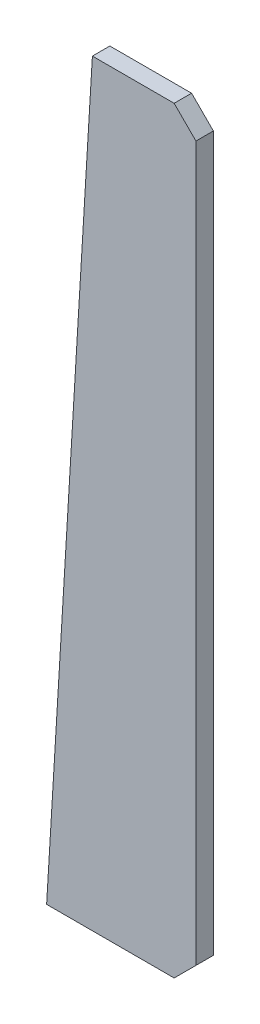
from build123d import *

# Parameters (mm, degrees)
EXTRUDE_1_DEPTH = 8
CHAMFER_1_SIZE  = 20


with BuildPart() as part:
    # 草图2 → 凸台-拉伸1 (new, symmetric)
    with BuildSketch(Plane.XY):
        Polygon((0, 0), (42, 695), (137, 695), (137, 0), align=None)
    extrude(amount=EXTRUDE_1_DEPTH, both=True)

    # 倒角1
    chamfer_1_edges = [part.edges().sort_by_distance(p)[0] for p in [
        (137, 695, 0),
        (137, 0, 0),
    ]]
    chamfer(chamfer_1_edges, length=CHAMFER_1_SIZE)


solid = part.part
